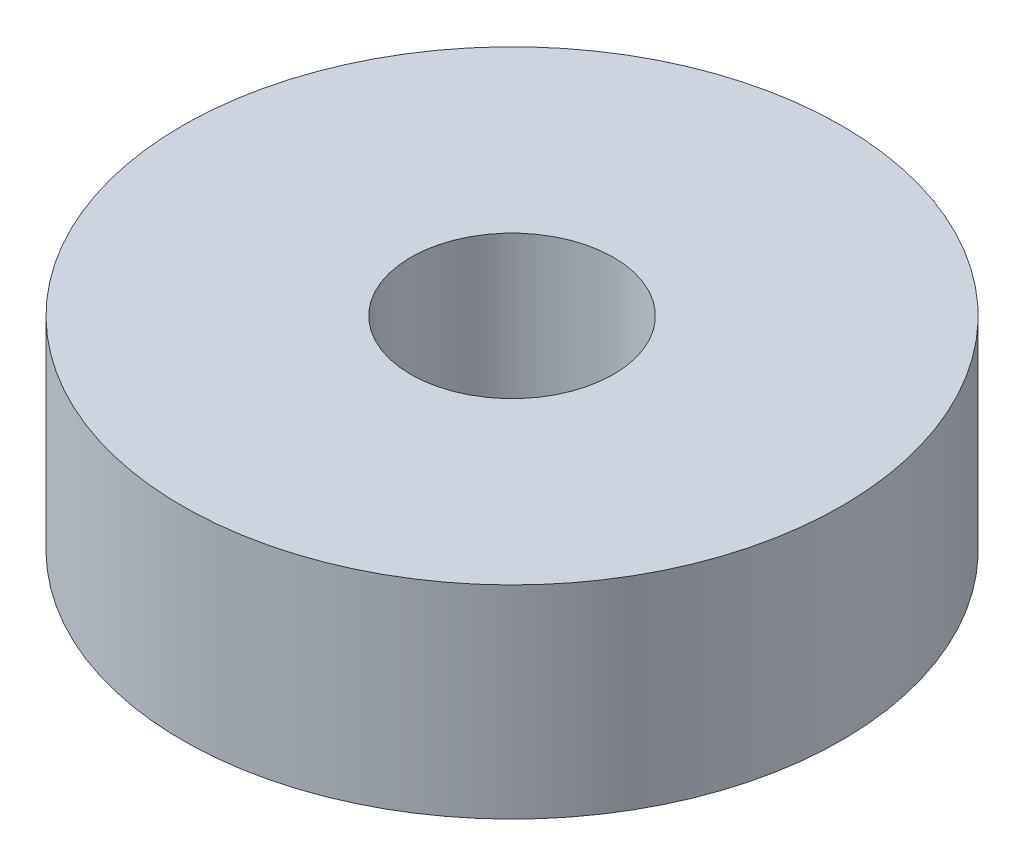
SolidWorks part; units mm, degrees
ref_plane "前视基准面" through (0, 0, 0) normal (0, 0, 1) x (1, 0, 0)
ref_plane "上视基准面" through (0, 0, 0) normal (0, 1, 0) x (1, 0, 0)
ref_plane "右视基准面" through (0, 0, 0) normal (1, 0, 0) x (0, 0, -1)
sketch "草图1" plane through (0, 0, 0) normal (0, 0, 1) x (1, 0, 0)
  line L0 (0, 0) -> (0, 2139.2592) construction
  line L2 (2, 1.6537) -> (6.5, 1.6537)
  line L3 (2, 1.6537) -> (2, -2.3463)
  line L4 (2, -2.3463) -> (6.5, -2.3463)
  line L5 (6.5, 1.6537) -> (6.5, -2.3463)
  dimension "D1" = 2
  dimension "D2" = 4
  dimension "D3" = 4.5
revolve "旋转1" add sketch "草图1" angle 360 about L0
